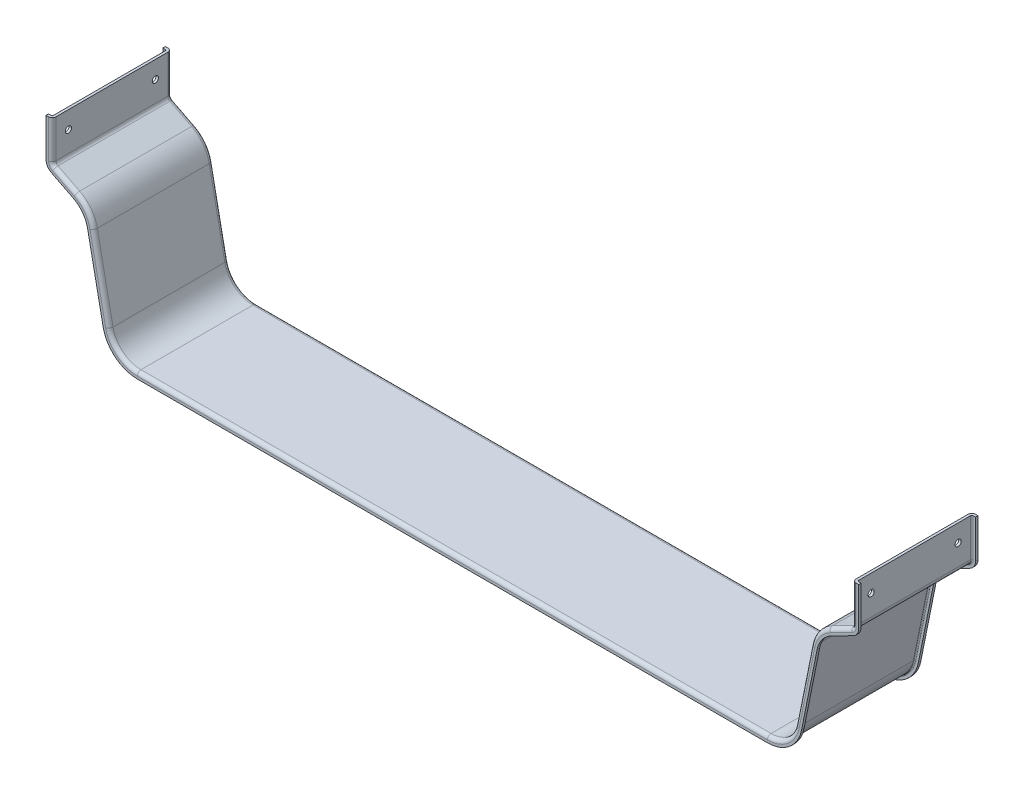
from build123d import *

# Parameters (mm, degrees)
SKETCH1_W                      = 1302.001638203
SKETCH1_H                      = 288
BOSS_EXTRUDE1_DEPTH            = 192
SKETCH2_W                      = 6
SKETCH2_H                      = 188
CUT_EXTRUDE1_DEPTH             = 1493.678808133
CUT_EXTRUDE2_DEPTH             = 184
SKETCH4_W                      = 1302.001638203
SKETCH4_H                      = 4
BOSS_EXTRUDE2_DEPTH            = 6
CUT_EXTRUDE3_DEPTH             = 184
SKETCH6_W                      = 4
SKETCH6_H                      = 294
BOSS_EXTRUDE3_DEPTH            = 6
SKETCH7_W                      = 4
SKETCH7_H                      = 288
BOSS_EXTRUDE4_DEPTH            = 6
SKETCH8_W                      = 1302.001638203
SKETCH8_H                      = 4
BOSS_EXTRUDE5_DEPTH            = 6
SKETCH9_W                      = 4
SKETCH9_H                      = 294
BOSS_EXTRUDE6_DEPTH            = 6
CUT_EXTRUDE4_DEPTH             = 1518.19698392
CUT_EXTRUDE5_REACH             = 1519.698
CUT_EXTRUDE6_DEPTH             = 1518.697825002
CUT_EXTRUDE7_DEPTH             = 1518.697825002
CUT_EXTRUDE8_DEPTH             = 1518.697825002
F_10_0_10_DIAMETER_HOLE1_D     = 10
F_10_0_10_DIAMETER_HOLE1_DEPTH = 4
F_10_0_10_DIAMETER_HOLE2_D     = 10
F_10_0_10_DIAMETER_HOLE2_DEPTH = 1302.001638202
FILLET1_R                      = 44
FILLET2_R                      = 10
FILLET3_R                      = 45.999999999
FILLET4_R                      = 50
FILLET5_R                      = 54
FILLET6_R                      = 2
FILLET7_R                      = 6
FILLET8_R                      = 16
FILLET9_R                      = 55.999999999


with BuildPart() as part:
    # Sketch1 → Boss-Extrude1 (new body)
    with BuildSketch(Plane.XY.offset(96)):
        with Locations((-810.481313615, 192.212549099)):
            Rectangle(SKETCH1_W, SKETCH1_H)
    extrude(amount=-BOSS_EXTRUDE1_DEPTH)

    # Sketch2 → Cut-Extrude1 (cut, through all)
    with BuildSketch(Plane(origin=(0, 336.212549099, 0), x_dir=(-1, 0, 0), z_dir=(0, 1, 0))):
        with Locations((162.480494514, -2)):
            Rectangle(SKETCH2_W, SKETCH2_H)
    extrude(amount=-CUT_EXTRUDE1_DEPTH, mode=Mode.SUBTRACT)

    # Sketch3 → Cut-Extrude2 (cut)
    with BuildSketch(Plane.XY.offset(92)):
        Polygon((-165.480494514, 48.212549099), (-165.480494514, 268.712549099), (-227.480494514, 237.212549099), (-265.480494514, 48.212549099), align=None)
    extrude(amount=-CUT_EXTRUDE2_DEPTH, mode=Mode.SUBTRACT)

    # Sketch4 → Boss-Extrude2 (add)
    with BuildSketch(Plane.XZ.offset(-48.212549099)):
        with Locations((-810.481313615, 94)):
            Rectangle(SKETCH4_W, SKETCH4_H)
    extrude(amount=BOSS_EXTRUDE2_DEPTH)

    # Sketch5 → Cut-Extrude3 (cut)
    with BuildSketch(Plane.XY.offset(92)):
        Polygon((-1461.482132717, 268.712549099), (-1461.482132717, 48.212549099), (-1361.482132717, 48.212549099), (-1399.482132717, 237.212549099), align=None)
    extrude(amount=-CUT_EXTRUDE3_DEPTH, mode=Mode.SUBTRACT)

    # Sketch6 → Boss-Extrude3 (add)
    with BuildSketch(Plane.ZY.offset(1461.482132717)):
        with Locations((94, 189.212549099)):
            Rectangle(SKETCH6_W, SKETCH6_H)
    extrude(amount=BOSS_EXTRUDE3_DEPTH)

    # Sketch7 → Boss-Extrude4 (add)
    with BuildSketch(Plane(origin=(-165.480494514, 0, 0), x_dir=(0, 0, -1), z_dir=(1, 0, 0))):
        with Locations((94, 192.212549099)):
            Rectangle(SKETCH7_W, SKETCH7_H)
    extrude(amount=BOSS_EXTRUDE4_DEPTH)

    # Sketch8 → Boss-Extrude5 (add)
    with BuildSketch(Plane.XZ.offset(-48.212549099)):
        with Locations((-810.481313615, -94)):
            Rectangle(SKETCH8_W, SKETCH8_H)
    extrude(amount=BOSS_EXTRUDE5_DEPTH)

    # Sketch9 → Boss-Extrude6 (add)
    with BuildSketch(Plane.ZY.offset(1461.482132717)):
        with Locations((-94, 189.212549099)):
            Rectangle(SKETCH9_W, SKETCH9_H)
    extrude(amount=BOSS_EXTRUDE6_DEPTH)

    # Sketch10 → Cut-Extrude4 (cut, through all)
    with BuildSketch(Plane(origin=(0, 0, 92), x_dir=(-1, 0, 0), z_dir=(0, 0, -1))):
        Polygon((222.171192902, 233.180034395), (159.480494514, 265.030953737), (159.480494514, 42.212549099), (260.566771956, 42.212549099), align=None)
    extrude(amount=-CUT_EXTRUDE4_DEPTH, mode=Mode.SUBTRACT)

    # Sketch11 → Cut-Extrude5 (cut, up to next)
    with BuildSketch(Plane.XY.offset(96), mode=Mode.PRIVATE) as cut_extrude5_sk1:
        Polygon((-1404.79143433, 233.180034395), (-1467.482132717, 265.030953737), (-1467.482132717, 42.212549099), (-1366.395855275, 42.212549099), align=None)
    cut_extrude5_tool1 = extrude(cut_extrude5_sk1.sketch, amount=-CUT_EXTRUDE5_REACH, mode=Mode.PRIVATE) & part.part
    add(cut_extrude5_tool1.solids().sort_by_distance((-1427.035862, 137.049675, 96))[0], mode=Mode.SUBTRACT)

    # Sketch12 → Cut-Extrude6 (cut, through all)
    with BuildSketch(Plane(origin=(0, 0, -96), x_dir=(-1, 0, 0), z_dir=(0, 0, -1))):
        Polygon((1457.482132717, 336.212549099), (169.480494514, 336.212549099), (169.480494514, 271.166946007), (231.020028923, 239.900892235), (268.756309553, 52.212549099), (1358.206317678, 52.212549099), (1395.942598308, 239.900892235), (1457.482132717, 271.166946007), align=None)
    extrude(amount=-CUT_EXTRUDE6_DEPTH, mode=Mode.SUBTRACT)

    # Sketch13 → Cut-Extrude7 (cut, through all)
    with BuildSketch(Plane(origin=(0, 0, -96), x_dir=(-1, 0, 0), z_dir=(0, 0, -1))):
        Polygon((1467.482132717, 265.030953737), (1404.79143433, 233.180034395), (1366.395855275, 42.212549099), (1467.482132717, 42.212549099), align=None)
    extrude(amount=-CUT_EXTRUDE7_DEPTH, mode=Mode.SUBTRACT)

    # Sketch14 → Cut-Extrude8 (cut, through all)
    with BuildSketch(Plane(origin=(0, 0, -96), x_dir=(-1, 0, 0), z_dir=(0, 0, -1))):
        Polygon((222.171192902, 233.180034395), (159.480494514, 265.030953737), (159.480494514, 42.212549099), (260.566771956, 42.212549099), align=None)
    extrude(amount=-CUT_EXTRUDE8_DEPTH, mode=Mode.SUBTRACT)

    # Ø10.0 (10) Diameter Hole1
    with Locations(Plane.ZY.offset(1461.482132717)):
        with Locations((-70, 308.212549099), (70, 308.212549099)):
            Hole(F_10_0_10_DIAMETER_HOLE1_D / 2, depth=F_10_0_10_DIAMETER_HOLE1_DEPTH)

    # Ø10.0 (10) Diameter Hole2
    with Locations(Plane(origin=(-165.480494514, 0, 0), x_dir=(0, 0, -1), z_dir=(1, 0, 0))):
        with Locations((70, 308.212549099), (-70, 308.212549099)):
            Hole(F_10_0_10_DIAMETER_HOLE2_D / 2, depth=F_10_0_10_DIAMETER_HOLE2_DEPTH)

    # Fillet1
    fillet1_edges = [part.edges().sort_by_distance(p)[0] for p in [
        (-222.171192902, 233.180034395, 94),
        (-1404.79143433, 233.180034395, 94),
        (-1404.79143433, 233.180034395, -94),
        (-222.171192902, 233.180034395, -94),
    ]]
    fillet(fillet1_edges, radius=FILLET1_R)

    # Fillet2
    fillet2_edges = [part.edges().sort_by_distance(p)[0] for p in [
        (-165.480494514, 268.712549099, 0),
        (-1461.482132717, 268.712549099, 0),
    ]]
    fillet(fillet2_edges, radius=FILLET2_R)

    # Fillet3
    fillet3_edges = [part.edges().sort_by_distance(p)[0] for p in [
        (-1358.206317678, 52.212549099, 0),
        (-268.756309553, 52.212549099, 0),
    ]]
    fillet(fillet3_edges, radius=FILLET3_R)

    # Fillet4
    fillet4_edges = [part.edges().sort_by_distance(p)[0] for p in [
        (-265.480494514, 48.212549099, 0),
        (-227.480494514, 237.212549099, 0),
        (-1399.482132717, 237.212549099, 0),
        (-1361.482132717, 48.212549099, 0),
    ]]
    fillet(fillet4_edges, radius=FILLET4_R)

    # Fillet5
    fillet5_edges = [part.edges().sort_by_distance(p)[0] for p in [
        (-1395.942598308, 239.900892235, 0),
        (-231.020028923, 239.900892235, 0),
    ]]
    fillet(fillet5_edges, radius=FILLET5_R)

    # Fillet6
    fillet6_edges = [part.edges().sort_by_distance(p)[0] for p in [
        (-1461.482132717, 305.530545234, -92),
        (-188.417527915, 257.059056323, 92),
        (-188.417527915, 257.059056323, -92),
        (-165.480494514, 305.530545234, 92),
        (-1460.005501102, 269.618609116, 92),
        (-1460.005501102, 269.618609116, -92),
        (-166.957126129, 269.618609116, 92),
        (-166.957126129, 269.618609116, -92),
        (-1438.545099316, 257.059056323, 92),
        (-1438.545099316, 257.059056323, -92),
        (-1382.130378776, 150.910404501, 92),
        (-813.481313616, 48.212549099, 92),
        (-244.832248455, 150.910404501, 92),
        (-223.0536514, 233.850278267, 92),
        (-1403.908975831, 233.850278267, 92),
        (-1382.130378776, 150.910404501, -92),
        (-244.832248455, 150.910404501, -92),
        (-813.481313616, 48.212549099, -92),
        (-223.0536514, 233.850278267, -92),
        (-1403.908975831, 233.850278267, -92),
        (-274.748409223, 59.529323213, 92),
        (-274.748409223, 59.529323213, -92),
        (-1352.214218008, 59.529323213, 92),
        (-1352.214218008, 59.529323213, -92),
        (-1461.482132717, 305.530545234, 92),
        (-165.480494514, 305.530545234, -92),
    ]]
    fillet(fillet6_edges, radius=FILLET6_R)

    # Fillet7
    fillet7_edges = [part.edges().sort_by_distance(p)[0] for p in [
        (-1457.482132717, 303.689747553, 96),
        (-1457.482132717, 271.166946007, 0),
        (-188.588221124, 261.458988133, 96),
        (-169.480494514, 303.689747553, 96),
        (-169.480494514, 271.166946007, 0),
        (-1457.482132717, 303.689747553, -96),
        (-169.480494514, 303.689747553, -96),
        (-188.588221124, 261.458988133, -96),
        (-813.481313616, 52.212549099, -96),
        (-813.481313616, 52.212549099, 96),
        (-1378.208856134, 151.698858788, -96),
        (-1378.208856134, 151.698858788, 96),
        (-277.282791085, 62.623981284, -96),
        (-277.282791085, 62.623981284, 96),
        (-1349.679836146, 62.623981284, -96),
        (-1349.679836146, 62.623981284, 96),
        (-248.753771097, 151.698858788, -96),
        (-248.753771097, 151.698858788, 96),
        (-1438.374406107, 261.458988133, -96),
        (-1400.723588872, 236.269639737, -96),
        (-226.23903836, 236.269639737, -96),
        (-1438.374406107, 261.458988133, 96),
        (-1400.723588872, 236.269639737, 96),
        (-226.23903836, 236.269639737, 96),
    ]]
    fillet(fillet7_edges, radius=FILLET7_R)

    # Fillet8
    fillet8_edges = [part.edges().sort_by_distance(p)[0] for p in [
        (-159.480494514, 265.030953737, 94),
        (-1467.482132717, 265.030953737, 94),
        (-1467.482132717, 265.030953737, -94),
        (-159.480494514, 265.030953737, -94),
    ]]
    fillet(fillet8_edges, radius=FILLET8_R)

    # Fillet9
    fillet9_edges = [part.edges().sort_by_distance(p)[0] for p in [
        (-260.566771956, 42.212549099, 94),
        (-1366.395855275, 42.212549099, 94),
        (-1366.395855275, 42.212549099, -94),
        (-260.566771956, 42.212549099, -94),
    ]]
    fillet(fillet9_edges, radius=FILLET9_R)


solid = part.part
